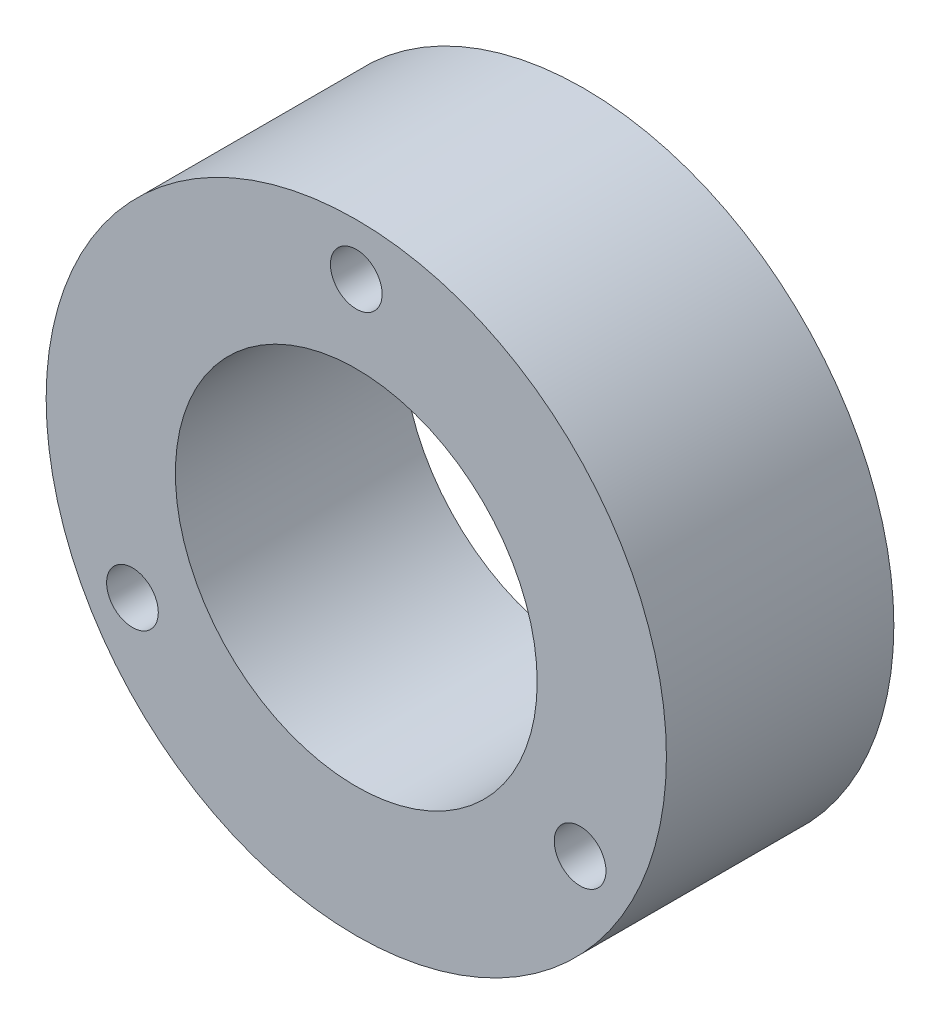
from build123d import *

# Parameters (mm, degrees)
SKETCH1_R           = 30
SKETCH1_R_2         = 17.5
SKETCH1_R_3         = 2.5
BOSS_EXTRUDE1_DEPTH = 22


with BuildPart() as part:
    # Sketch1 → Boss-Extrude1 (new body)
    with BuildSketch(Plane.XY):
        Circle(SKETCH1_R)
        Circle(SKETCH1_R_2, mode=Mode.SUBTRACT)
        with Locations((0, 25)):
            Circle(SKETCH1_R_3, mode=Mode.SUBTRACT)
        with Locations((21.650635095, -12.5)):
            Circle(SKETCH1_R_3, mode=Mode.SUBTRACT)
        with Locations((-21.650635095, -12.5)):
            Circle(SKETCH1_R_3, mode=Mode.SUBTRACT)
    extrude(amount=BOSS_EXTRUDE1_DEPTH)


solid = part.part
